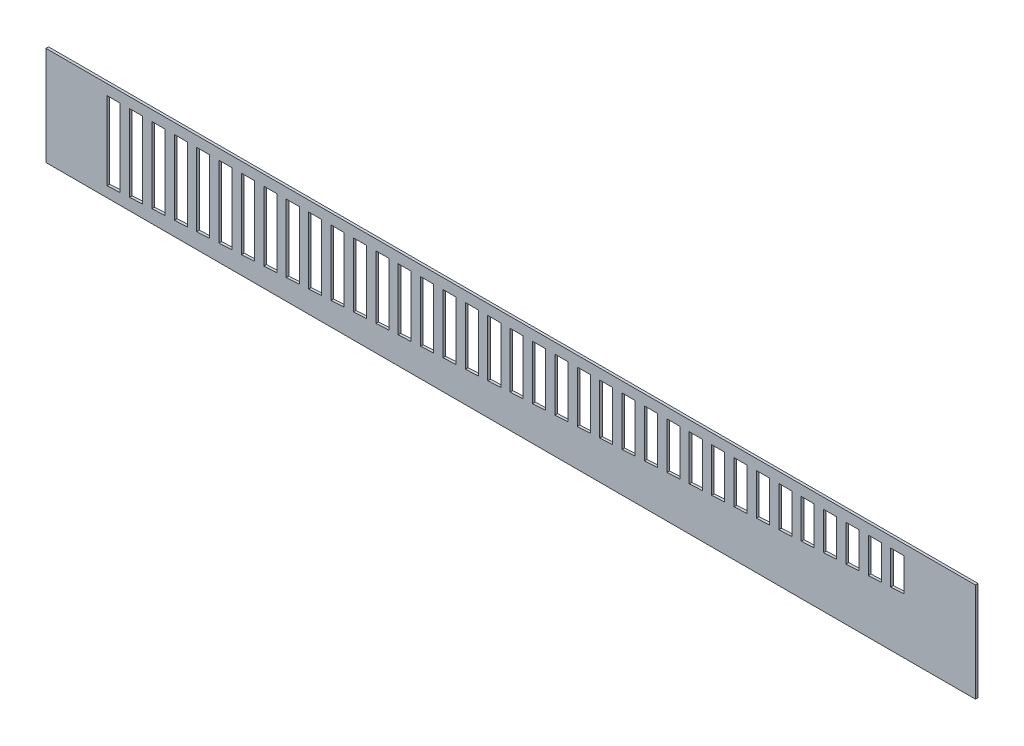
SolidWorks part; units mm, degrees
material "AISI 316 stainless steel plate (SS)"
ref_plane "Front Plane" through (0, 0, 0) normal (0, 0, 1) x (1, 0, 0)
ref_plane "Top Plane" through (0, 0, 0) normal (0, 1, 0) x (1, 0, 0)
ref_plane "Right Plane" through (0, 0, 0) normal (1, 0, 0) x (0, 0, -1)
other "Configuration Table"
sketch "Sketch1" plane through (0, 0, 0) normal (0, 0, 1) x (1, 0, 0)
  line L1 (-89.25, -9.5) -> (89.25, -9.5)
  line L2 (-89.25, -9.5) -> (-89.25, 9.5)
  line L3 (-89.25, 9.5) -> (89.25, 9.5)
  line L4 (89.25, -9.5) -> (89.25, 9.5)
  line L5 (-89.25, -9.5) -> (89.25, 9.5) construction
  line L6 (-89.25, 9.5) -> (89.25, -9.5) construction
  point P0 (0, 0)
  dimension "D1" = 19
  dimension "D2" = 178.5
extrude "Boss-Extrude1" add sketch "Sketch1" along normal blind 0.5
sketch "Sketch2" plane through (0, 0, 0.5) normal (0, 0, 1) x (1, 0, 0)
  line L1 (-77.51, 7.5) -> (-75.01, 7.5)
  line L2 (-77.51, 7.5) -> (-77.51, -7.5)
  line L4 (-75.01, 7.5) -> (-75.01, -7.3585)
  line L183 (-89.25, 9.5) -> (-89.25, -9.5) construction
  line L184 (-70.71, 7.5) -> (-70.71, -7.1151)
  line L185 (-73.21, 7.5) -> (-70.71, 7.5)
  line L186 (-73.21, 7.5) -> (-73.21, -7.2566)
  line L188 (-66.41, 7.5) -> (-66.41, -6.8716)
  line L189 (-68.91, 7.5) -> (-66.41, 7.5)
  line L190 (-68.91, 7.5) -> (-68.91, -7.0132)
  line L192 (-62.11, 7.5) -> (-62.11, -6.6282)
  line L193 (-64.61, 7.5) -> (-62.11, 7.5)
  line L194 (-64.61, 7.5) -> (-64.61, -6.7697)
  line L196 (-57.81, 7.5) -> (-57.81, -6.3848)
  line L197 (-60.31, 7.5) -> (-57.81, 7.5)
  line L198 (-60.31, 7.5) -> (-60.31, -6.5263)
  line L200 (-53.51, 7.5) -> (-53.51, -6.1414)
  line L201 (-56.01, 7.5) -> (-53.51, 7.5)
  line L202 (-56.01, 7.5) -> (-56.01, -6.2829)
  line L204 (-49.21, 7.5) -> (-49.21, -5.898)
  line L205 (-51.71, 7.5) -> (-49.21, 7.5)
  line L206 (-51.71, 7.5) -> (-51.71, -6.0395)
  line L208 (-44.91, 7.5) -> (-44.91, -5.6545)
  line L209 (-47.41, 7.5) -> (-44.91, 7.5)
  line L210 (-47.41, 7.5) -> (-47.41, -5.7961)
  line L212 (-40.61, 7.5) -> (-40.61, -5.4111)
  line L213 (-43.11, 7.5) -> (-40.61, 7.5)
  line L214 (-43.11, 7.5) -> (-43.11, -5.5526)
  line L216 (-36.31, 7.5) -> (-36.31, -5.1677)
  line L217 (-38.81, 7.5) -> (-36.31, 7.5)
  line L218 (-38.81, 7.5) -> (-38.81, -5.3092)
  line L220 (-32.01, 7.5) -> (-32.01, -4.9243)
  line L221 (-34.51, 7.5) -> (-32.01, 7.5)
  line L222 (-34.51, 7.5) -> (-34.51, -5.0658)
  line L224 (-27.71, 7.5) -> (-27.71, -4.6809)
  line L225 (-30.21, 7.5) -> (-27.71, 7.5)
  line L226 (-30.21, 7.5) -> (-30.21, -4.8224)
  line L228 (-23.41, 7.5) -> (-23.41, -4.4375)
  line L229 (-25.91, 7.5) -> (-23.41, 7.5)
  line L230 (-25.91, 7.5) -> (-25.91, -4.579)
  line L232 (-19.11, 7.5) -> (-19.11, -4.194)
  line L233 (-21.61, 7.5) -> (-19.11, 7.5)
  line L234 (-21.61, 7.5) -> (-21.61, -4.3356)
  line L236 (-14.81, 7.5) -> (-14.81, -3.9506)
  line L237 (-17.31, 7.5) -> (-14.81, 7.5)
  line L238 (-17.31, 7.5) -> (-17.31, -4.0921)
  line L240 (-10.51, 7.5) -> (-10.51, -3.7072)
  line L241 (-13.01, 7.5) -> (-10.51, 7.5)
  line L242 (-13.01, 7.5) -> (-13.01, -3.8487)
  line L244 (-6.21, 7.5) -> (-6.21, -3.4638)
  line L245 (-8.71, 7.5) -> (-6.21, 7.5)
  line L246 (-8.71, 7.5) -> (-8.71, -3.6053)
  line L248 (-1.91, 7.5) -> (-1.91, -3.2204)
  line L249 (-4.41, 7.5) -> (-1.91, 7.5)
  line L250 (-4.41, 7.5) -> (-4.41, -3.3619)
  line L252 (2.39, 7.5) -> (2.39, -2.9769)
  line L253 (-0.11, 7.5) -> (2.39, 7.5)
  line L254 (-0.11, 7.5) -> (-0.11, -3.1185)
  line L256 (6.69, 7.5) -> (6.69, -2.7335)
  line L257 (4.19, 7.5) -> (6.69, 7.5)
  line L258 (4.19, 7.5) -> (4.19, -2.875)
  line L260 (10.99, 7.5) -> (10.99, -2.4901)
  line L261 (8.49, 7.5) -> (10.99, 7.5)
  line L262 (8.49, 7.5) -> (8.49, -2.6316)
  line L264 (15.29, 7.5) -> (15.29, -2.2467)
  line L265 (12.79, 7.5) -> (15.29, 7.5)
  line L266 (12.79, 7.5) -> (12.79, -2.3882)
  line L268 (19.59, 7.5) -> (19.59, -2.0033)
  line L269 (17.09, 7.5) -> (19.59, 7.5)
  line L270 (17.09, 7.5) -> (17.09, -2.1448)
  line L272 (23.89, 7.5) -> (23.89, -1.7598)
  line L273 (21.39, 7.5) -> (23.89, 7.5)
  line L274 (21.39, 7.5) -> (21.39, -1.9014)
  line L276 (28.19, 7.5) -> (28.19, -1.5164)
  line L277 (25.69, 7.5) -> (28.19, 7.5)
  line L278 (25.69, 7.5) -> (25.69, -1.6579)
  line L280 (32.49, 7.5) -> (32.49, -1.273)
  line L281 (29.99, 7.5) -> (32.49, 7.5)
  line L282 (29.99, 7.5) -> (29.99, -1.4145)
  line L284 (36.79, 7.5) -> (36.79, -1.0296)
  line L285 (34.29, 7.5) -> (36.79, 7.5)
  line L286 (34.29, 7.5) -> (34.29, -1.1711)
  line L288 (41.09, 7.5) -> (41.09, -0.7862)
  line L289 (38.59, 7.5) -> (41.09, 7.5)
  line L290 (38.59, 7.5) -> (38.59, -0.9277)
  line L292 (45.39, 7.5) -> (45.39, -0.5428)
  line L293 (42.89, 7.5) -> (45.39, 7.5)
  line L294 (42.89, 7.5) -> (42.89, -0.6843)
  line L296 (49.69, 7.5) -> (49.69, -0.2993)
  line L297 (47.19, 7.5) -> (49.69, 7.5)
  line L298 (47.19, 7.5) -> (47.19, -0.4409)
  line L300 (53.99, 7.5) -> (53.99, -0.0559)
  line L301 (51.49, 7.5) -> (53.99, 7.5)
  line L302 (51.49, 7.5) -> (51.49, -0.1974)
  line L304 (58.29, 7.5) -> (58.29, 0.1875)
  line L305 (55.79, 7.5) -> (58.29, 7.5)
  line L306 (55.79, 7.5) -> (55.79, 0.046)
  line L308 (62.59, 7.5) -> (62.59, 0.4309)
  line L309 (60.09, 7.5) -> (62.59, 7.5)
  line L310 (60.09, 7.5) -> (60.09, 0.2894)
  line L312 (66.89, 7.5) -> (66.89, 0.6743)
  line L313 (64.39, 7.5) -> (66.89, 7.5)
  line L314 (64.39, 7.5) -> (64.39, 0.5328)
  line L316 (71.19, 7.5) -> (71.19, 0.9178)
  line L317 (68.69, 7.5) -> (71.19, 7.5)
  line L318 (68.69, 7.5) -> (68.69, 0.7762)
  line L320 (75.49, 7.5) -> (75.49, 1.1612)
  line L321 (72.99, 7.5) -> (75.49, 7.5)
  line L322 (72.99, 7.5) -> (72.99, 1.0197)
  line L394 (-77.51, -7.5) -> (-75.01, -7.3585)
  line L395 (-89.25, -9.5) -> (89.25, -9.5) construction
  line L396 (-73.21, -7.2566) -> (-70.71, -7.1151)
  line L397 (-68.91, -7.0132) -> (-66.41, -6.8716)
  line L398 (-64.61, -6.7697) -> (-62.11, -6.6282)
  line L399 (-60.31, -6.5263) -> (-57.81, -6.3848)
  line L400 (-56.01, -6.2829) -> (-53.51, -6.1414)
  line L401 (-51.71, -6.0395) -> (-49.21, -5.898)
  line L402 (-47.41, -5.7961) -> (-44.91, -5.6545)
  line L403 (-43.11, -5.5526) -> (-40.61, -5.4111)
  line L404 (-38.81, -5.3092) -> (-36.31, -5.1677)
  line L405 (-34.51, -5.0658) -> (-32.01, -4.9243)
  line L406 (-30.21, -4.8224) -> (-27.71, -4.6809)
  line L407 (-25.91, -4.579) -> (-23.41, -4.4375)
  line L408 (-21.61, -4.3356) -> (-19.11, -4.194)
  line L409 (-17.31, -4.0921) -> (-14.81, -3.9506)
  line L410 (-13.01, -3.8487) -> (-10.51, -3.7072)
  line L411 (-8.71, -3.6053) -> (-6.21, -3.4638)
  line L412 (-4.41, -3.3619) -> (-1.91, -3.2204)
  line L413 (-0.11, -3.1185) -> (2.39, -2.9769)
  line L414 (4.19, -2.875) -> (6.69, -2.7335)
  line L415 (8.49, -2.6316) -> (10.99, -2.4901)
  line L416 (12.79, -2.3882) -> (15.29, -2.2467)
  line L417 (17.09, -2.1448) -> (19.59, -2.0033)
  line L418 (21.39, -1.9014) -> (23.89, -1.7598)
  line L419 (25.69, -1.6579) -> (28.19, -1.5164)
  line L420 (29.99, -1.4145) -> (32.49, -1.273)
  line L421 (34.29, -1.1711) -> (36.79, -1.0296)
  line L422 (38.59, -0.9277) -> (41.09, -0.7862)
  line L423 (42.89, -0.6843) -> (45.39, -0.5428)
  line L424 (47.19, -0.4409) -> (49.69, -0.2993)
  line L425 (51.49, -0.1974) -> (53.99, -0.0559)
  line L426 (55.79, 0.046) -> (58.29, 0.1875)
  line L427 (60.09, 0.2894) -> (62.59, 0.4309)
  line L428 (72.99, 1.0197) -> (75.49, 1.1612)
  line L429 (68.69, 0.7762) -> (71.19, 0.9178)
  line L430 (64.39, 0.5328) -> (66.89, 0.6743)
  dimension "D1" = 11.74
  dimension "D2" = 2.5
  dimension "D3" = 36
  dimension "D4" = 3.24
extrude "Cut-Extrude1" cut sketch "Sketch2" against normal blind 147.56
